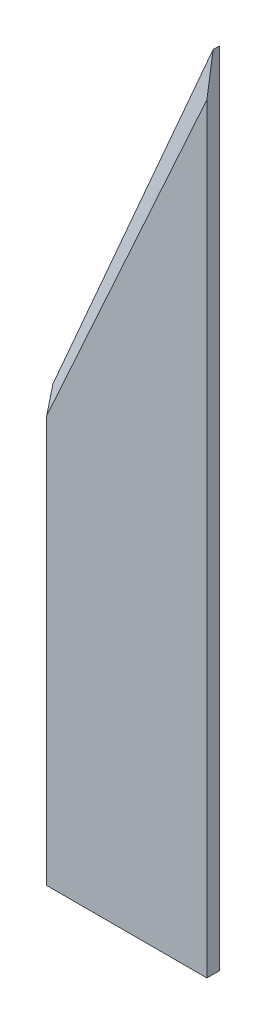
SolidWorks part; units mm, degrees
ref_plane "Front Plane" through (0, 0, 0) normal (0, 0, 1) x (1, 0, 0)
ref_plane "Top Plane" through (0, 0, 0) normal (0, 1, 0) x (1, 0, 0)
ref_plane "Right Plane" through (0, 0, 0) normal (1, 0, 0) x (0, 0, -1)
other "Configuration Table"
sketch "Sketch1" plane through (0, 0, 0) normal (0, 1, 0) x (1, 0, 0)
  line L1 (-6.5, -0.5) -> (6.5, -0.5)
  line L2 (-6.5, -0.5) -> (-6.5, 0.5)
  line L3 (-6.5, 0.5) -> (6.5, 0.5)
  line L4 (6.5, -0.5) -> (6.5, 0.5)
  line L5 (0, 0.5) -> (0, -0.5) construction
  line L6 (-6.5, 0) -> (6.5, 0) construction
  point P0 (0, 0)
  dimension "D1" = 1
  dimension "D2" = 13
extrude "Boss-Extrude1" add sketch "Sketch1" along normal blind 35
sketch "Sketch3" plane through (0, 0, 0.5) normal (0, 0, 1) x (1, 0, 0)
  line L0 (6.5, 35) -> (-6.5, 5)
  line L1 (-6.5, 35) -> (-6.5, 0) construction
  line L2 (-6.5, 5) -> (-6.5, 35)
  line L3 (-6.5, 35) -> (6.5, 35)
  dimension "D1" = 30
extrude "Cut-Extrude2" cut sketch "Sketch3" against normal through all
sketch "Sketch6" plane through (-6.5, 0, 0) normal (-1, 0, 0) x (0, 0, 1)
  line L0 (0, 5) -> (0.5, 3.0275)
  line L1 (-0.5, 5) -> (0.5, 5) construction
  line L2 (0.5, 5) -> (0.5, 0) construction
  line L3 (0.5, 3.0275) -> (0.5, 5)
  line L4 (0.5, 5) -> (0, 5)
sketch "Sketch7" plane through (6.5, 0, 0) normal (1, 0, 0) x (0, 0, -1)
  line L0 (0, 35) -> (-0.5, 31.7309)
  line L1 (-0.5, 35) -> (0.5, 35) construction
  line L2 (-0.5, 35) -> (-0.5, 0) construction
  line L3 (-0.5, 31.7309) -> (-0.5, 35)
  line L4 (-0.5, 35) -> (0, 35)
loft "Cut-Loft2" cut profiles "Sketch7", "Sketch6"
sketch "Sketch8" plane through (0, 0, 0) normal (0, -1, 0) x (1, 0, 0)
  line L4 (6.5, -0.5) -> (6.5, 0.5)
  line L5 (6.5, 0.5) -> (-6.5, 0.5)
  line L6 (-6.5, 0.5) -> (-6.5, -0.5)
  line L7 (-6.5, -0.5) -> (6.5, -0.5)
  line L8 (6.5, -0.5) -> (6.5, 0.5)
  line L9 (6.5, 0.5) -> (-6.5, 0.5)
  line L10 (-6.5, 0.5) -> (-6.5, -0.5)
  line L11 (-6.5, -0.5) -> (6.5, -0.5)
  dimension "D1" = 0
extrude "Boss-Extrude2" add sketch "Sketch8" along normal blind 30
